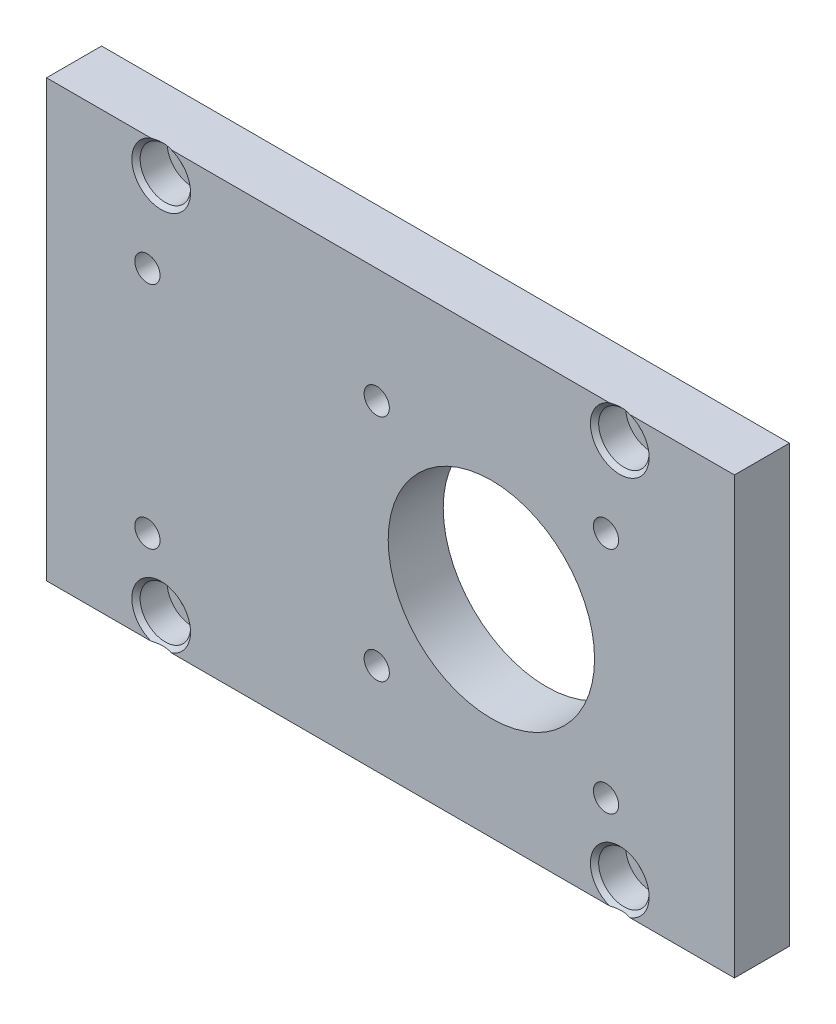
from build123d import *

# Parameters (mm, degrees)
SKETCH_1_W               = 150
SKETCH_1_H               = 95
EXTRUDE_1_DEPTH          = 12
HOLE_WIZARD_1_AT_2_COUNT = 2
HOLE_WIZARD_1_AT_2_PITCH = 100
HOLE_WIZARD_1_AT_3_COUNT = 2
HOLE_WIZARD_1_AT_3_PITCH = 83
HOLE_WIZARD_1_AT_4_COUNT = 2
HOLE_WIZARD_1_AT_4_PITCH = 129.957685421
HOLE_WIZARD_2_AT_2_COUNT = 2
HOLE_WIZARD_2_AT_2_PITCH = 50
HOLE_WIZARD_2_AT_3_COUNT = 2
HOLE_WIZARD_2_AT_3_PITCH = 100
HOLE_WIZARD_2_AT_4_COUNT = 2
HOLE_WIZARD_2_AT_4_PITCH = 111.803398875
HOLE_WIZARD_2_AT_5_COUNT = 2
HOLE_WIZARD_2_AT_5_PITCH = 70.710678119
HOLE_WIZARD_2_AT_6_COUNT = 2
HOLE_WIZARD_2_AT_6_PITCH = 50
SKETCH_9_R               = 22.5
CUT_EXTRUDE_1_DEPTH      = 90.583759689


with BuildPart() as part:
    # 草图1 → 凸台-拉伸1 (new body)
    with BuildSketch(Plane.XY):
        Rectangle(SKETCH_1_W, SKETCH_1_H)
    extrude(amount=EXTRUDE_1_DEPTH)

    # 草图6 → 打孔尺寸(%根据)内六角圆柱头螺钉的类型1 (revolve, cut)
    with BuildSketch(Plane(origin=(-50, -41.5, 12), x_dir=(0, -1, 0), z_dir=(1, 0, 0))):
        Polygon((0, 0), (0, 12), (3.3, 12), (3.3, 6.8), (5.5, 6.8), (5.5, 0.9), (6.4, 0), align=None)
    hole_wizard_1 = revolve(axis=Axis((-50, -41.5, 18.35), (0, 0, -1)), mode=Mode.SUBTRACT)

    # 打孔尺寸(%根据)内六角圆柱头螺钉的类型1 at 2: 打孔尺寸(%根据)内六角圆柱头螺钉的类型1 ×2
    with Locations(*[(i * HOLE_WIZARD_1_AT_2_PITCH, 0, 0) for i in range(1, HOLE_WIZARD_1_AT_2_COUNT)]):
        add(hole_wizard_1, mode=Mode.SUBTRACT)

    # 打孔尺寸(%根据)内六角圆柱头螺钉的类型1 at 3: 打孔尺寸(%根据)内六角圆柱头螺钉的类型1 ×2
    with Locations(*[(0, i * HOLE_WIZARD_1_AT_3_PITCH, 0) for i in range(1, HOLE_WIZARD_1_AT_3_COUNT)]):
        add(hole_wizard_1, mode=Mode.SUBTRACT)

    # 打孔尺寸(%根据)内六角圆柱头螺钉的类型1 at 4: 打孔尺寸(%根据)内六角圆柱头螺钉的类型1 ×2
    with Locations(*[Vector(0.7694812328797624, 0.6386694232902033, 0) * (i * HOLE_WIZARD_1_AT_4_PITCH) for i in range(1, HOLE_WIZARD_1_AT_4_COUNT)]):
        add(hole_wizard_1, mode=Mode.SUBTRACT)

    # 草图8 → 打孔尺寸(%根据)内六角圆柱头螺钉的类型2 (revolve, cut)
    with BuildSketch(Plane(origin=(-53, -27.5, 0), x_dir=(0, 1, 0), z_dir=(1, 0, 0))):
        Polygon((0, 0), (0, 12), (2.75, 12), (2.75, 5.7), (5, 5.7), (5, 0.025), (5.025, 0), align=None)
    hole_wizard_2 = revolve(axis=Axis((-53, -27.5, -6.35), (0, 0, 1)), mode=Mode.SUBTRACT)

    # 打孔尺寸(%根据)内六角圆柱头螺钉的类型2 at 2: 打孔尺寸(%根据)内六角圆柱头螺钉的类型2 ×2
    with Locations(*[(i * HOLE_WIZARD_2_AT_2_PITCH, 0, 0) for i in range(1, HOLE_WIZARD_2_AT_2_COUNT)]):
        add(hole_wizard_2, mode=Mode.SUBTRACT)

    # 打孔尺寸(%根据)内六角圆柱头螺钉的类型2 at 3: 打孔尺寸(%根据)内六角圆柱头螺钉的类型2 ×2
    with Locations(*[(i * HOLE_WIZARD_2_AT_3_PITCH, 0, 0) for i in range(1, HOLE_WIZARD_2_AT_3_COUNT)]):
        add(hole_wizard_2, mode=Mode.SUBTRACT)

    # 打孔尺寸(%根据)内六角圆柱头螺钉的类型2 at 4: 打孔尺寸(%根据)内六角圆柱头螺钉的类型2 ×2
    with Locations(*[Vector(0.8944271909999156, 0.4472135954999584, 0) * (i * HOLE_WIZARD_2_AT_4_PITCH) for i in range(1, HOLE_WIZARD_2_AT_4_COUNT)]):
        add(hole_wizard_2, mode=Mode.SUBTRACT)

    # 打孔尺寸(%根据)内六角圆柱头螺钉的类型2 at 5: 打孔尺寸(%根据)内六角圆柱头螺钉的类型2 ×2
    with Locations(*[Vector(0.7071067811865471, 0.7071067811865479, 0) * (i * HOLE_WIZARD_2_AT_5_PITCH) for i in range(1, HOLE_WIZARD_2_AT_5_COUNT)]):
        add(hole_wizard_2, mode=Mode.SUBTRACT)

    # 打孔尺寸(%根据)内六角圆柱头螺钉的类型2 at 6: 打孔尺寸(%根据)内六角圆柱头螺钉的类型2 ×2
    with Locations(*[(0, i * HOLE_WIZARD_2_AT_6_PITCH, 0) for i in range(1, HOLE_WIZARD_2_AT_6_COUNT)]):
        add(hole_wizard_2, mode=Mode.SUBTRACT)

    # 草图9 → 切除-拉伸1 (cut, through all)
    with BuildSketch(Plane(origin=(0, 0, 0), x_dir=(-1, 0, 0), z_dir=(0, 0, -1))):
        with Locations((-22, -2.5)):
            Circle(SKETCH_9_R)
    extrude(amount=-CUT_EXTRUDE_1_DEPTH, mode=Mode.SUBTRACT)


solid = part.part
